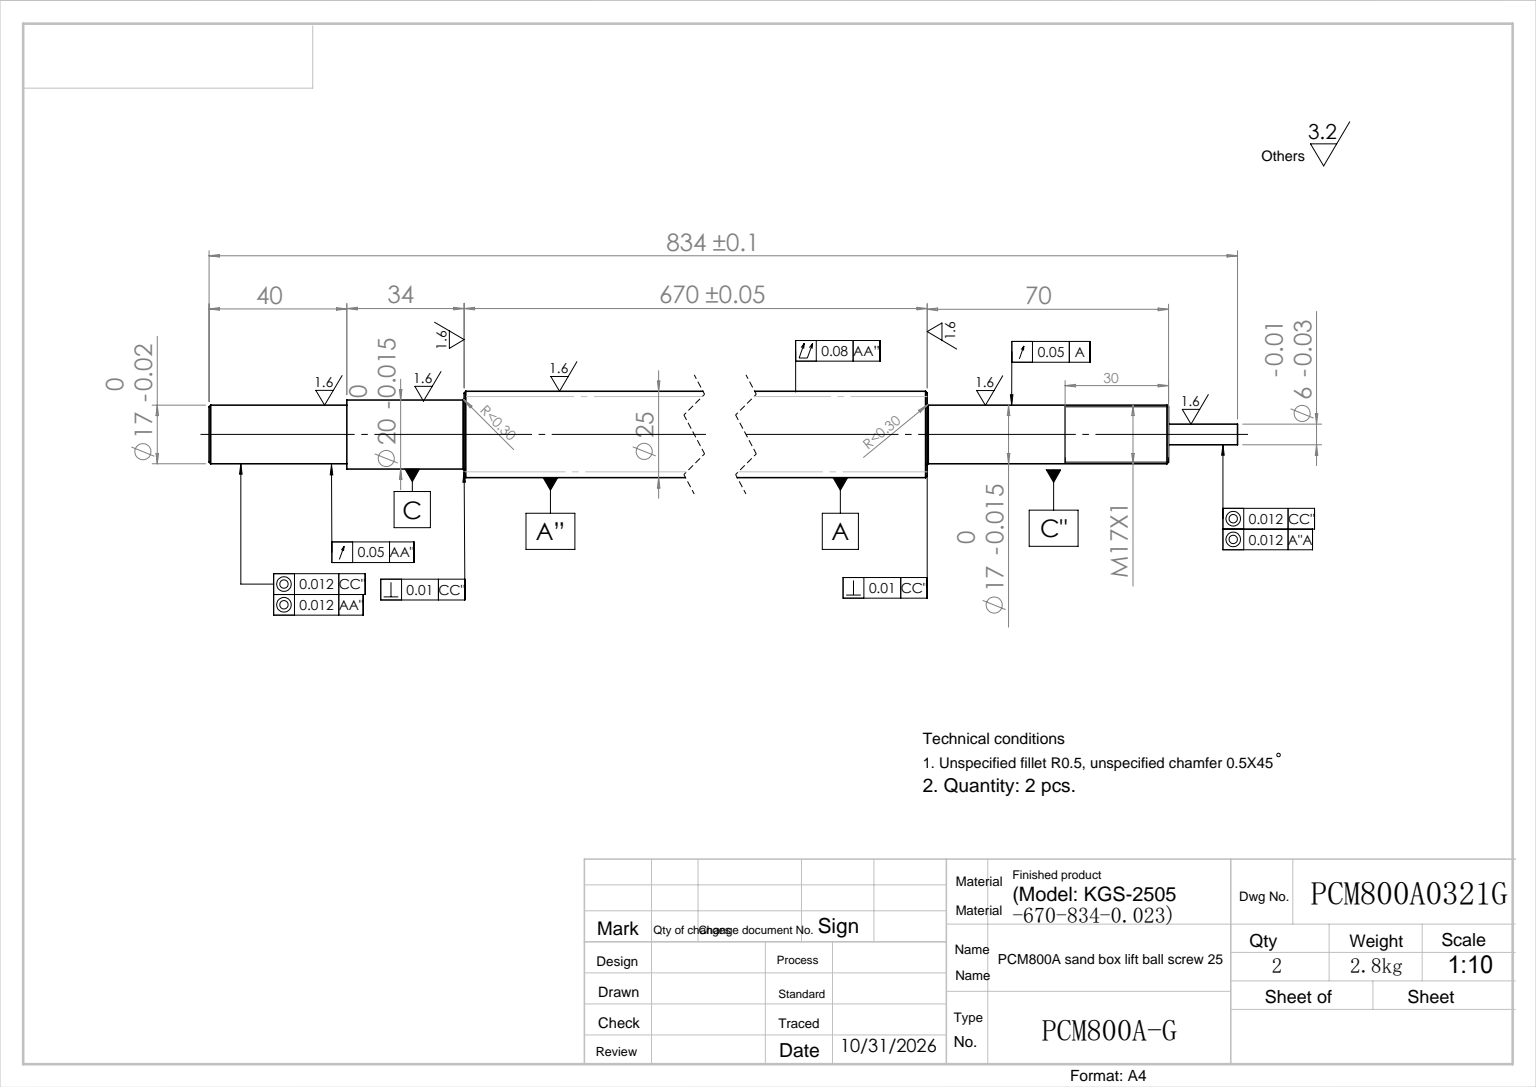
SolidWorks part; units mm, degrees
ref_plane "前视基准面" through (0, 0, 0) normal (0, 0, 1) x (1, 0, 0)
ref_plane "上视基准面" through (0, 0, 0) normal (0, 1, 0) x (1, 0, 0)
ref_plane "右视基准面" through (0, 0, 0) normal (1, 0, 0) x (0, 0, -1)
sketch "草图1" plane through (0, 0, 0) normal (0, 1, 0) x (1, 0, 0)
  circle A0 centre (0, 0) radius 8.5
extrude "拉伸1" add sketch "草图1" along normal blind 70
cosmetic thread "装饰螺纹线1" parameters "D1"=30, "D2"=16
sketch "草图2" plane through (0, 70, 0) normal (0, 1, 0) x (-1, 0, 0)
  circle A0 centre (0, 0) radius 12.5
extrude "拉伸2" add sketch "草图2" along normal blind 670
sketch "草图3" plane through (0, 740, 0) normal (0, 1, 0) x (-1, 0, 0)
  circle A0 centre (0, 0) radius 10
extrude "拉伸3" add sketch "草图3" along normal blind 34
sketch "草图4" plane through (0, 774, 0) normal (0, 1, 0) x (-1, 0, 0)
  circle A0 centre (0, 0) radius 8.5
extrude "拉伸4" add sketch "草图4" along normal blind 40
chamfer "倒角1" distance 0.5 angle 45 4 edges at (0, 0, 8.5) (0, 70, 12.5) (0, 740, 12.5) (0, 814, 8.5)
fillet "圆角1" radius 0.3 1 edges at (0, 70, 8.5)
fillet "圆角2" radius 0.3 1 edges at (0, 740, 10)
sketch "草图5" plane through (0, 0, 0) normal (0, -1, 0) x (1, 0, 0)
  circle A0 centre (0, 0) radius 3
extrude "拉伸5" add sketch "草图5" along normal blind 20
